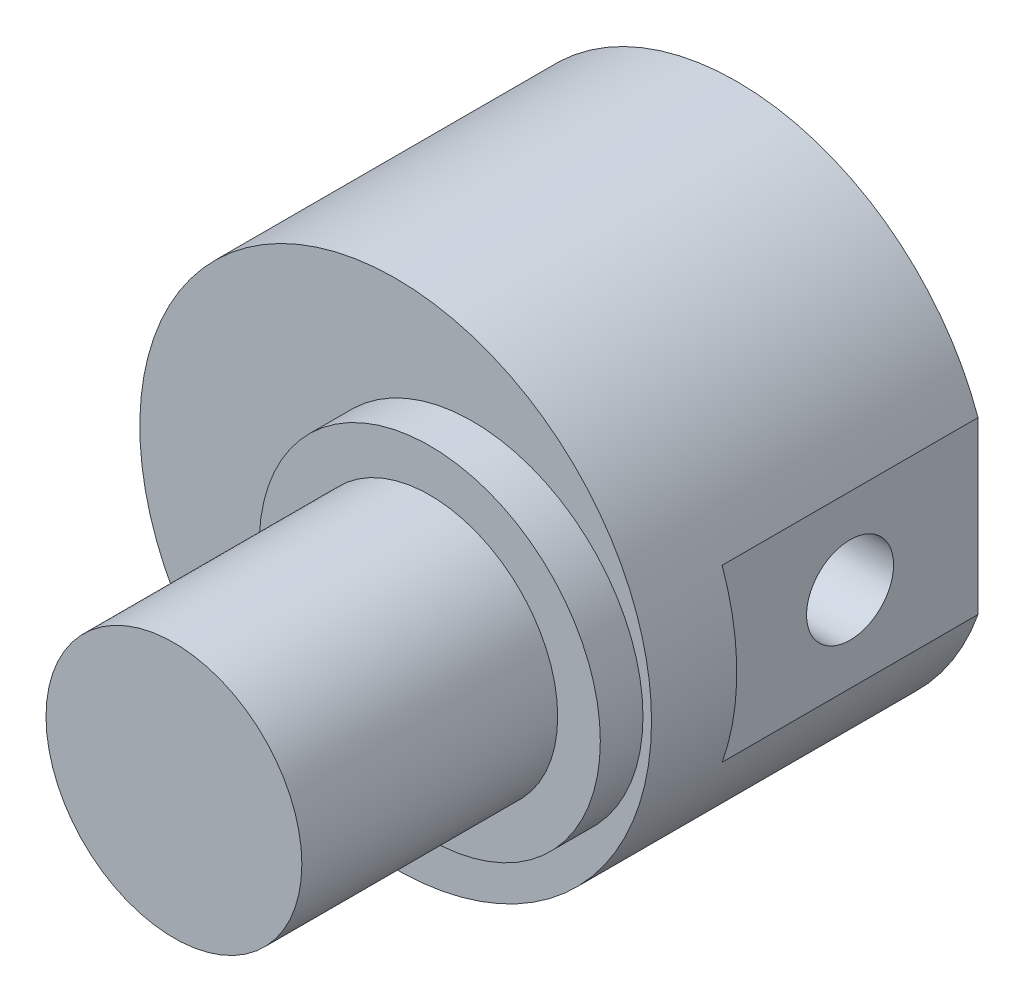
from build123d import *

# Parameters (mm, degrees)
SKETCH_1_R              = 30
EXTRUDE_1_DEPTH         = 40
SKETCH_2_R              = 20
EXTRUDE_2_DEPTH         = 5
SKETCH_3_R              = 15
EXTRUDE_3_DEPTH         = 30
SKETCH_5_R              = 18
CUT_EXTRUDE_1_DEPTH     = 30
HOLE_WIZARD_M12_1_D     = 10.2
HOLE_WIZARD_M12_1_DEPTH = 29.25
HOLE_WIZARD_M12_1_TIP   = 3.064389157


with BuildPart() as part:
    # 草图1 → 凸台-拉伸1 (new body)
    with BuildSketch(Plane.XY):
        Circle(SKETCH_1_R)
    extrude(amount=EXTRUDE_1_DEPTH)

    # 草图2 → 凸台-拉伸2 (add)
    with BuildSketch(Plane.XY.offset(40)):
        with Locations((9, 0)):
            Circle(SKETCH_2_R)
    extrude(amount=EXTRUDE_2_DEPTH)

    # 草图3 → 凸台-拉伸3 (add)
    with BuildSketch(Plane.XY.offset(45)):
        with Locations((9, 0)):
            Circle(SKETCH_3_R)
    extrude(amount=EXTRUDE_3_DEPTH)

    # 草图5 → 切除-拉伸1 (cut)
    with BuildSketch(Plane(origin=(0, 0, 0), x_dir=(-1, 0, 0), z_dir=(0, 0, -1))):
        Circle(SKETCH_5_R)
        Polygon((-30.259977001, 10), (-28.284271247, 10), (-28.284271247, -10), (-32.220348536, -10), (-32.220348536, 10), align=None)
    extrude(amount=-CUT_EXTRUDE_1_DEPTH, mode=Mode.SUBTRACT)

    # M12 螺纹孔1
    with Locations(Plane(origin=(28.284271247, 0, 0), x_dir=(0, 0, -1), z_dir=(1, 0, 0))):
        with Locations((-15, 0)):
            Hole(HOLE_WIZARD_M12_1_D / 2, depth=HOLE_WIZARD_M12_1_DEPTH)
            with Locations((0, 0, -(HOLE_WIZARD_M12_1_DEPTH + HOLE_WIZARD_M12_1_TIP / 2))):  # 118° drill point
                Cone(0, HOLE_WIZARD_M12_1_D / 2, HOLE_WIZARD_M12_1_TIP, mode=Mode.SUBTRACT)


solid = part.part
